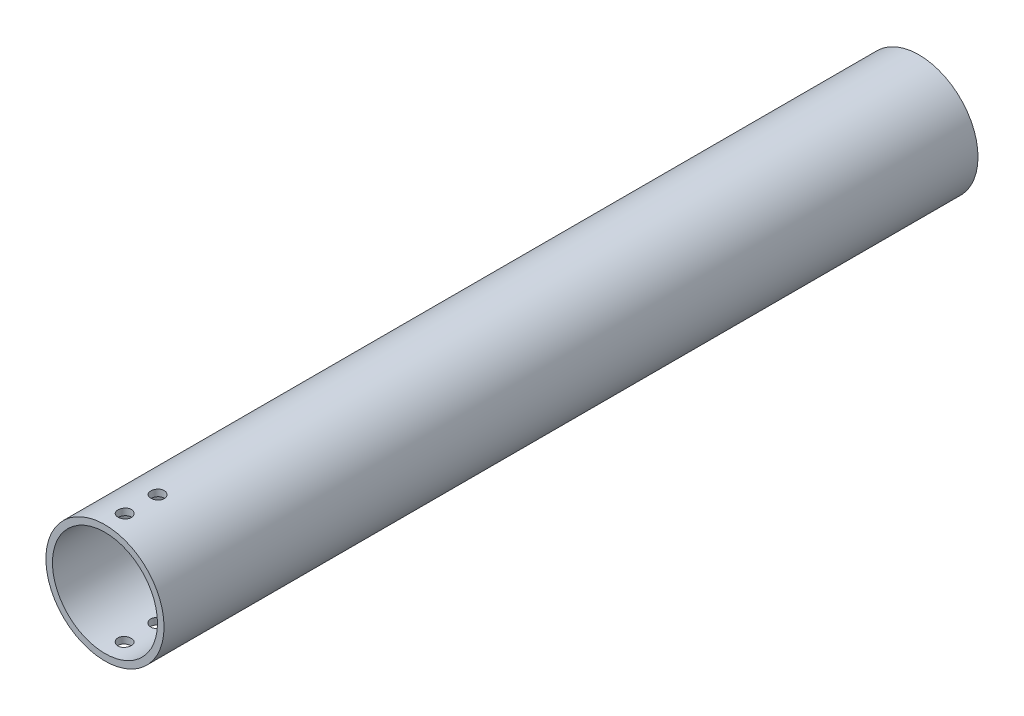
SolidWorks part; units mm, degrees
ref_plane "前视基准面" through (0, 0, 0) normal (0, 0, 1) x (1, 0, 0)
ref_plane "上视基准面" through (0, 0, 0) normal (0, 1, 0) x (1, 0, 0)
ref_plane "右视基准面" through (0, 0, 0) normal (1, 0, 0) x (0, 0, -1)
sketch "草图1" plane through (0, 0, 0) normal (0, 0, 1) x (1, 0, 0)
  circle A0 centre (0, 0) radius 45
  circle A1 centre (0, 0) radius 40
  dimension "D1" = 90
  dimension "D2" = 5
extrude "凸台-拉伸1" add sketch "草图1" along normal blind 40
sketch "草图2" plane through (0, 0, 40) normal (0, 0, 1) x (1, 0, 0)
  circle A0 centre (0, 0) radius 40 construction
  circle A1 centre (0, 0) radius 40
  circle A3 centre (0, 0) radius 50
  dimension "D1" = 10
extrude "凸台-拉伸2" add sketch "草图2" along normal blind 30
sketch "草图3" plane through (0, 0, 70) normal (0, 0, 1) x (1, 0, 0)
  circle A2 centre (0, 0) radius 40 construction
  circle A3 centre (0, 0) radius 40
  circle A4 centre (0, 0) radius 45
  dimension "D1" = 5
extrude "凸台-拉伸3" add sketch "草图3" along normal blind 550
sketch "草图4" plane through (0, 0, 0) normal (0, 1, 0) x (1, 0, 0)
  line L0 (0, -620) -> (0, -605) construction
  line L1 (-45, -620) -> (45, -620) construction
  line L2 (0, -605) -> (0, -580) construction
  circle A2 centre (0, -605) radius 5.1
  circle A3 centre (0, -580) radius 5.1
  dimension "D3" = 10.2
  dimension "D1" = 25
  dimension "D2" = 15
extrude "切除-拉伸1" cut sketch "草图4" against normal mid plane 182
sketch "草图5" plane through (0, 0, 40) normal (0, 0, -1) x (-1, 0, 0)
  circle A0 centre (0, 0) radius 45 construction
  circle A1 centre (0, 0) radius 50
  circle A2 centre (0, 0) radius 50
  circle A3 centre (0, 0) radius 45
  dimension "D1" = 0
extrude "切除-拉伸2" cut sketch "草图5" against normal blind 117
